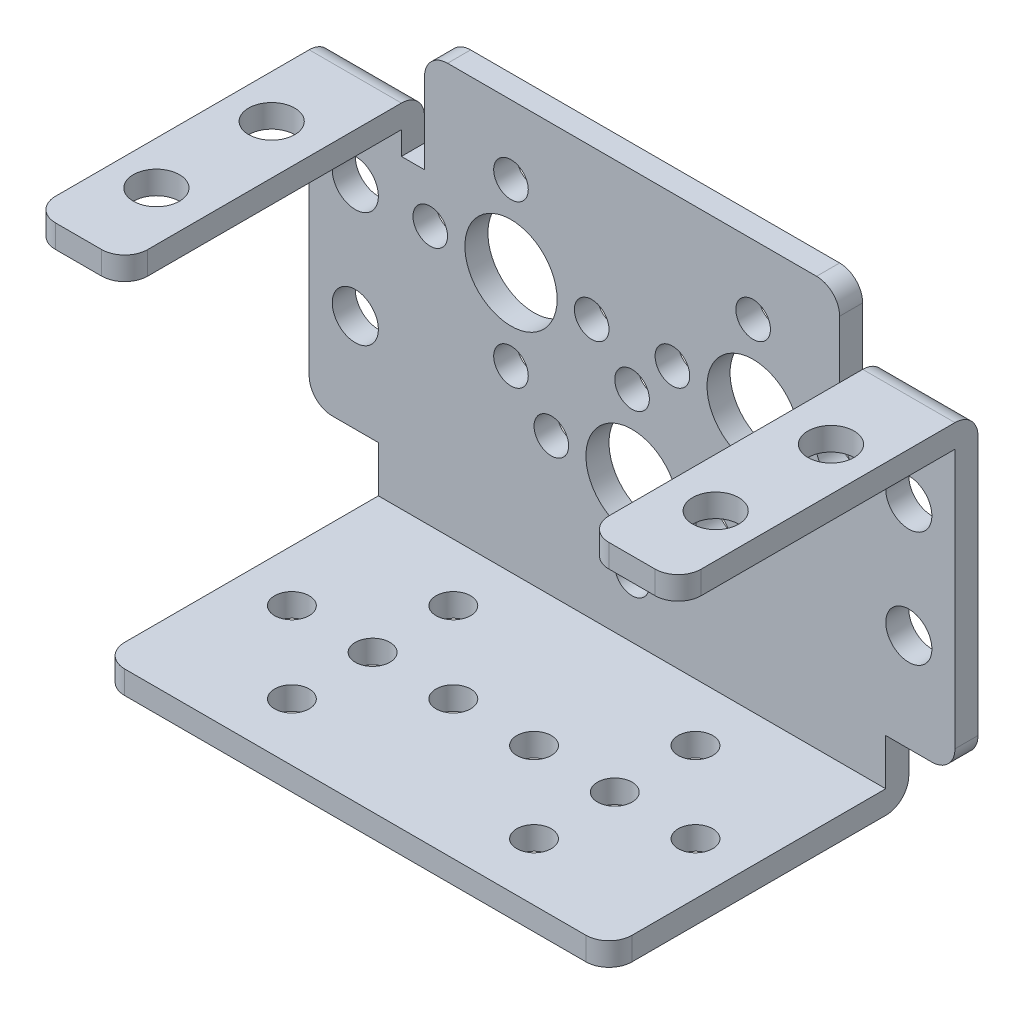
SolidWorks part; units mm, degrees
ref_plane "Front Plane" through (0, 0, 0) normal (0, 0, 1) x (1, 0, 0)
ref_plane "Top Plane" through (0, 0, 0) normal (0, 1, 0) x (1, 0, 0)
ref_plane "Right Plane" through (0, 0, 0) normal (1, 0, 0) x (0, 0, -1)
sketch "Sketch3" plane through (0, 0, 0) normal (0, 0, 1) x (1, 0, 0)
  line L0 (9.413, 70.4955) -> (172.0083, 70.4955) construction
  line L1 (-28, 18.745) -> (28, 18.745)
  line L2 (-28, 18.745) -> (-28, -18.745)
  line L3 (-28, -18.745) -> (28, -18.745)
  line L4 (28, 18.745) -> (28, -18.745)
  dimension "D1" = 56
  dimension "D2" = 37.49
  dimension "D3" = 28
  dimension "D4" = 18.745
extrude "Boss-Extrude1" add sketch "Sketch3" along normal blind 2
sketch "Sketch4" plane through (0, 0, 2) normal (0, 0, 1) x (1, 0, 0)
  line L0 (28, -18.745) -> (28, 18.745) construction
  line L1 (-28, -18.745) -> (28, -18.745)
  line L2 (-28, -18.745) -> (-28, -16.745)
  line L3 (-28, -16.745) -> (28, -16.745)
  line L4 (28, -18.745) -> (28, -16.745)
  dimension "D1" = 2
extrude "Boss-Extrude2" add sketch "Sketch4" along normal blind 24
sketch "Sketch5" plane through (0, 0, 2) normal (0, 0, 1) x (1, 0, 0)
  line L0 (-28, 18.745) -> (-28, -16.745) construction
  line L1 (-28, 11.755) -> (-20, 11.755)
  line L2 (-28, 11.755) -> (-28, 13.755)
  line L3 (-28, 13.755) -> (-20, 13.755)
  line L4 (-20, 11.755) -> (-20, 13.755)
  line L5 (-28, -18.745) -> (28, -18.745) construction
  line L6 (0, 0) -> (0, 20.1135) construction
  dimension "D1" = 2
  dimension "D2" = 32.5
  dimension "D3" = 8
extrude "Boss-Extrude3" add sketch "Sketch5" along normal blind 24
pattern_linear "LinPattern1" count 2 spacing 48 along (1, 0, 0) of "Boss-Extrude3"
sketch "Sketch6" plane through (0, 0, 2) normal (0, 0, 1) x (1, 0, 0)
  line L2 (-28, -18.745) -> (-22, -18.745)
  line L3 (-28, -18.745) -> (-28, -12.745)
  line L4 (-28, -12.745) -> (-22, -12.745)
  line L5 (-22, -18.745) -> (-22, -12.745)
  dimension "D1" = 6
  dimension "D2" = 6
extrude "Cut-Extrude1" cut sketch "Sketch6" against normal through all both and the other way through all
pattern_linear "LinPattern2" count 2 spacing 50 along (1, 0, 0) of "Cut-Extrude1"
sketch "Sketch7" plane through (0, 0, 2) normal (0, 0, 1) x (1, 0, 0)
  line L0 (-28, 18.745) -> (-28, 13.755)
  line L1 (-28, 13.755) -> (-20, 13.755)
  line L2 (-20, 13.755) -> (-20, 11.755)
  line L3 (-20, 11.755) -> (-20, 9.745)
  line L4 (-20, 9.745) -> (-18, 9.745)
  line L5 (-18, 9.745) -> (-18, 18.745)
  line L6 (28, 18.745) -> (-28, 18.745) construction
  line L7 (-18, 18.745) -> (-28, 18.745)
  dimension "D1" = 9
  dimension "D2" = 2
extrude "Cut-Extrude2" cut sketch "Sketch7" against normal blind 23.5
sketch "Sketch8" plane through (0, 0, 2) normal (0, 0, 1) x (1, 0, 0)
  line L0 (28, 13.755) -> (28, 18.745)
  line L1 (28, 18.745) -> (18, 18.745)
  line L2 (28, 18.745) -> (-18, 18.745) construction
  line L3 (18, 18.745) -> (18, 9.745)
  line L4 (18, 9.745) -> (20, 9.745)
  line L5 (20, 9.745) -> (20, 13.755)
  line L6 (20, 13.755) -> (28, 13.755)
  dimension "D1" = 2
  dimension "D2" = 9
extrude "Cut-Extrude3" cut sketch "Sketch8" against normal blind 23.5
sketch "Sketch9" plane through (0, 0, 2) normal (0, 0, 1) x (1, 0, 0)
  line L0 (-22, -12.745) -> (-28, -12.745) construction
  line L1 (-10.5, -14.381) -> (-10.5, 39.891) construction
  line L2 (-20.8924, 5.755) -> (-0.1076, 5.755) construction
  line L3 (-18, 9.745) -> (-18, 18.745) construction
  line L4 (-18, 18.745) -> (18, 18.745) construction
  line L5 (18, 18.745) -> (18, 12.2979) construction
  line L6 (18, 18.745) -> (18, 9.745) construction
  line L7 (0, 18.745) -> (0, -9.2021) construction
  line L8 (-28, 11.755) -> (-28, -12.745) construction
  line L9 (22, -16.745) -> (-22, -16.745) construction
  circle A0 centre (-24, 5.755) radius 2
  circle A1 centre (-24, -4.245) radius 2
  circle A2 centre (-10.5, 5.755) radius 4
  circle A3 centre (0, -4.745) radius 4
  circle A4 centre (0, 2.255) radius 1.5
  circle A5 centre (0, -11.745) radius 1.5
  circle A6 centre (-10.5, -1.245) radius 1.5
  circle A7 centre (-10.5, 12.755) radius 1.5
  circle A8 centre (-17.5, 5.755) radius 1.5
  circle A9 centre (-3.5, 5.755) radius 1.5
  circle A10 centre (-7, -4.745) radius 1.5
  circle A11 centre (7, -4.745) radius 1.5
  circle A12 centre (10.5, 12.755) radius 1.5
  circle A13 centre (3.5, 5.755) radius 1.5
  circle A14 centre (10.5, -1.245) radius 1.5
  circle A15 centre (10.5, 5.755) radius 4
  circle A16 centre (17.5, 5.755) radius 1.5
  circle A17 centre (24, -4.245) radius 2
  circle A18 centre (24, 5.755) radius 2
  dimension "D1" = 4
  dimension "D2" = 4
  dimension "D6" = 8
  dimension "D7" = 8
  dimension "D9" = 3
  dimension "D10" = 3
  dimension "D11" = 7
  dimension "D16" = 7
  dimension "D17" = 0
  dimension "D19" = 3
  dimension "D20" = 3
  dimension "D21" = 3
  dimension "D22" = 3
  dimension "D3" = 18.5
  dimension "D23" = 4
  dimension "D24" = 3
  dimension "D4" = 10
  dimension "D5" = 10.5
  dimension "D8" = 7
  dimension "D12" = 7
  dimension "D13" = 7
  dimension "D14" = 7
  dimension "D15" = 7
  dimension "D25" = 12
extrude "Cut-Extrude4" cut sketch "Sketch9" against normal blind 23.5
sketch "Sketch11" plane through (0, -16.745, 0) normal (0, 1, 0) x (1, 0, 0)
  line L0 (-22, -2) -> (-22, -26) construction
  line L1 (-22, -26) -> (22, -26) construction
  line L2 (-22, 0) -> (-22, -26) construction
  line L3 (-22, -14) -> (22, -14) construction
  line L4 (22, 0) -> (22, -26) construction
  line L5 (0, -26) -> (0, -2) construction
  line L6 (-1.5, -2) -> (1.5, -2) construction
  line L7 (0, -26) -> (-22, -26) construction
  circle A0 centre (-10.5, -14) radius 1.5
  circle A1 centre (-17.5, -14) radius 1.5
  circle A2 centre (-10.5, -21) radius 1.5
  circle A3 centre (-3.5, -14) radius 1.5
  circle A4 centre (-10.5, -7) radius 1.5
  circle A5 centre (10.5, -21) radius 1.5
  circle A6 centre (3.5, -14) radius 1.5
  circle A7 centre (10.5, -7) radius 1.5
  circle A8 centre (10.5, -14) radius 1.5
  circle A9 centre (17.5, -14) radius 1.5
  dimension "D1" = 3
  dimension "D2" = 3
  dimension "D3" = 3
  dimension "D4" = 3
  dimension "D10" = 3
  dimension "D5" = 7
  dimension "D6" = 7
  dimension "D7" = 7
  dimension "D8" = 7
  dimension "D9" = 7
extrude "Cut-Extrude5" cut sketch "Sketch11" against normal through all
fillet "Fillet1" radius 2 10 edges at (-24, 13.755, 0) (-18, 18.745, 1) (24, 13.755, 0) (18, 18.745, 1) (-28, 12.755, 26) (28, 12.755, 26) (0, -18.745, 0) (-28, -12.745, 1) (28, -12.745, 1)
sketch "Sketch12" plane through (0, 13.755, 0) normal (0, 1, 0) x (1, 0, 0)
  line L0 (0, 6.4055) -> (0, -31.5866) construction
  line L2 (-20, -24) -> (-20, -2) construction
  line L3 (-28, 0) -> (28, 0) construction
  line L4 (28, 0) -> (1, 0) construction
  line L7 (-10.5, -14) -> (-31.6786, -14) construction
  circle A0 centre (-24.25, -19) radius 2
  circle A1 centre (-24.25, -9) radius 2
  dimension "D2" = 4
  dimension "D3" = 4
  dimension "D4" = 4.25
  dimension "D5" = 5
  dimension "D1" = 5
  dimension "D7" = 4.25
extrude "Cut-Extrude6" cut sketch "Sketch12" against normal blind 23.5
mirror "Mirror2" about plane through (0, 0, 0) normal (1, 0, 0) of "Cut-Extrude6"
